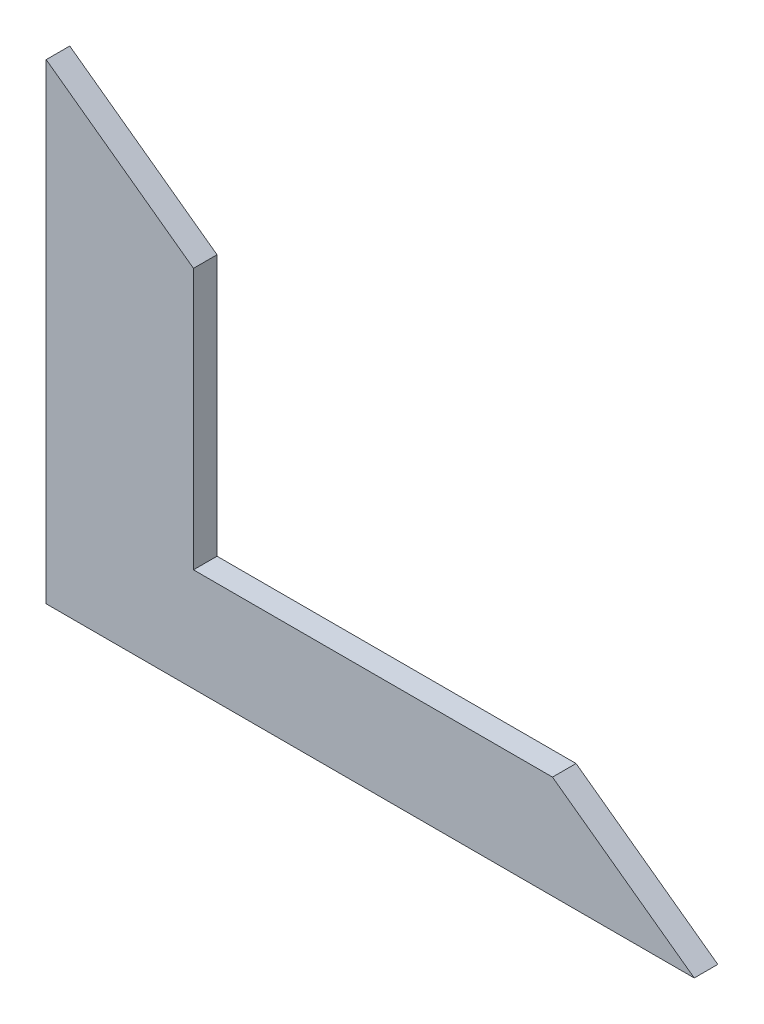
SolidWorks part; units mm, degrees
ref_plane "前视基准面" through (0, 0, 0) normal (0, 0, 1) x (1, 0, 0)
ref_plane "上视基准面" through (0, 0, 0) normal (0, 1, 0) x (1, 0, 0)
ref_plane "右视基准面" through (0, 0, 0) normal (1, 0, 0) x (0, 0, -1)
sketch "草图1" plane through (0, 0, 0) normal (0, 0, 1) x (1, 0, 0)
  line L0 (-140, 40) -> (-140, -120)
  line L1 (-140, -120) -> (80, -120)
  line L2 (80, -120) -> (31.875, -85)
  line L3 (31.875, -85) -> (-90, -85)
  line L4 (-90, -85) -> (-90, 3.6364)
  line L5 (-90, 3.6364) -> (-140, 40)
  dimension "D1" = 160
  dimension "D2" = 220
  dimension "D3" = 80
  dimension "D4" = 40
  dimension "D5" = 35
  dimension "D6" = 50
extrude "凸台-拉伸1" add sketch "草图1" along normal blind 8
hole_wizard "M4 螺纹孔1" positions "草图2" profile "草图3" tap size "M4" standard "ISO"
sketch "草图2" plane through (0, -120, 0) normal (0, -1, 0) x (-1, 0, 0)
  line L0 (140, -4) -> (-80, -4) construction
  line L1 (140, -8) -> (140, 0) construction
  line L2 (-80, -8) -> (-80, 0) construction
  line L4 (30, 0) -> (30, -8) construction
  line L5 (140, 0) -> (-80, 0) construction
  line L6 (140, -8) -> (-80, -8) construction
  point P0 (112.5, -4)
  point P2 (57.5, -4)
  point P4 (2.5, -4)
  point P6 (-52.5, -4)
  dimension "D1" = 27.5
  dimension "D2" = 27.5
  dimension "D3" = 55
  dimension "D4" = 55
sketch "草图3" plane through (-112.5, -120, 4) normal (1, 0, 0) x (0, 0, -1)
  line L0 (0, 0) -> (0, 15.9914)
  line L1 (0, 15.9914) -> (1.65, 15)
  line L2 (1.65, 15) -> (1.65, 0)
  line L5 (1.65, 0) -> (0, 0)
  line L10 (0, 15.9914) -> (-1.65, 15) construction
  line L11 (0, -6.35) -> (0, 107.95) construction
  dimension "螺纹孔钻头直径" = 3.3
  dimension "螺纹孔钻头深度" = 15
  dimension "导头角度" = 118
cosmetic thread "孔螺蚊线1" parameters "D1"=13, "D2"=4
cosmetic thread "孔螺蚊线2" parameters "D1"=13, "D2"=4
cosmetic thread "孔螺蚊线3" parameters "D1"=13, "D2"=4
cosmetic thread "孔螺蚊线4" parameters "D1"=13, "D2"=4
hole_wizard "M4 螺纹孔2" positions "草图4" profile "草图5" tap size "M4" standard "ISO"
sketch "草图4" plane through (-140, 0, 0) normal (-1, 0, 0) x (0, 0, 1)
  line L0 (4, -120) -> (4, 40) construction
  line L1 (8, -120) -> (0, -120) construction
  line L2 (8, 40) -> (0, 40) construction
  line L4 (0, -40) -> (8, -40) construction
  line L5 (0, 40) -> (0, -120) construction
  line L6 (8, 40) -> (8, -120) construction
  point P0 (4, 20)
  point P2 (4, -40)
  point P4 (4, -100)
  dimension "D1" = 60
  dimension "D2" = 60
sketch "草图5" plane through (-140, 20, 4) normal (0, 1, 0) x (0, 0, 1)
  line L0 (0, 0) -> (0, 16.0914)
  line L1 (0, 16.0914) -> (1.65, 15.1)
  line L2 (1.65, 15.1) -> (1.65, 0)
  line L5 (1.65, 0) -> (0, 0)
  line L10 (0, 16.0914) -> (-1.65, 15.1) construction
  line L11 (0, -6.35) -> (0, 107.95) construction
  dimension "螺纹孔钻头直径" = 3.3
  dimension "螺纹孔钻头深度" = 15.1
  dimension "导头角度" = 118
cosmetic thread "孔螺蚊线5" parameters "D1"=13, "D2"=4
cosmetic thread "孔螺蚊线6" parameters "D1"=13, "D2"=4
cosmetic thread "孔螺蚊线7" parameters "D1"=13, "D2"=4
